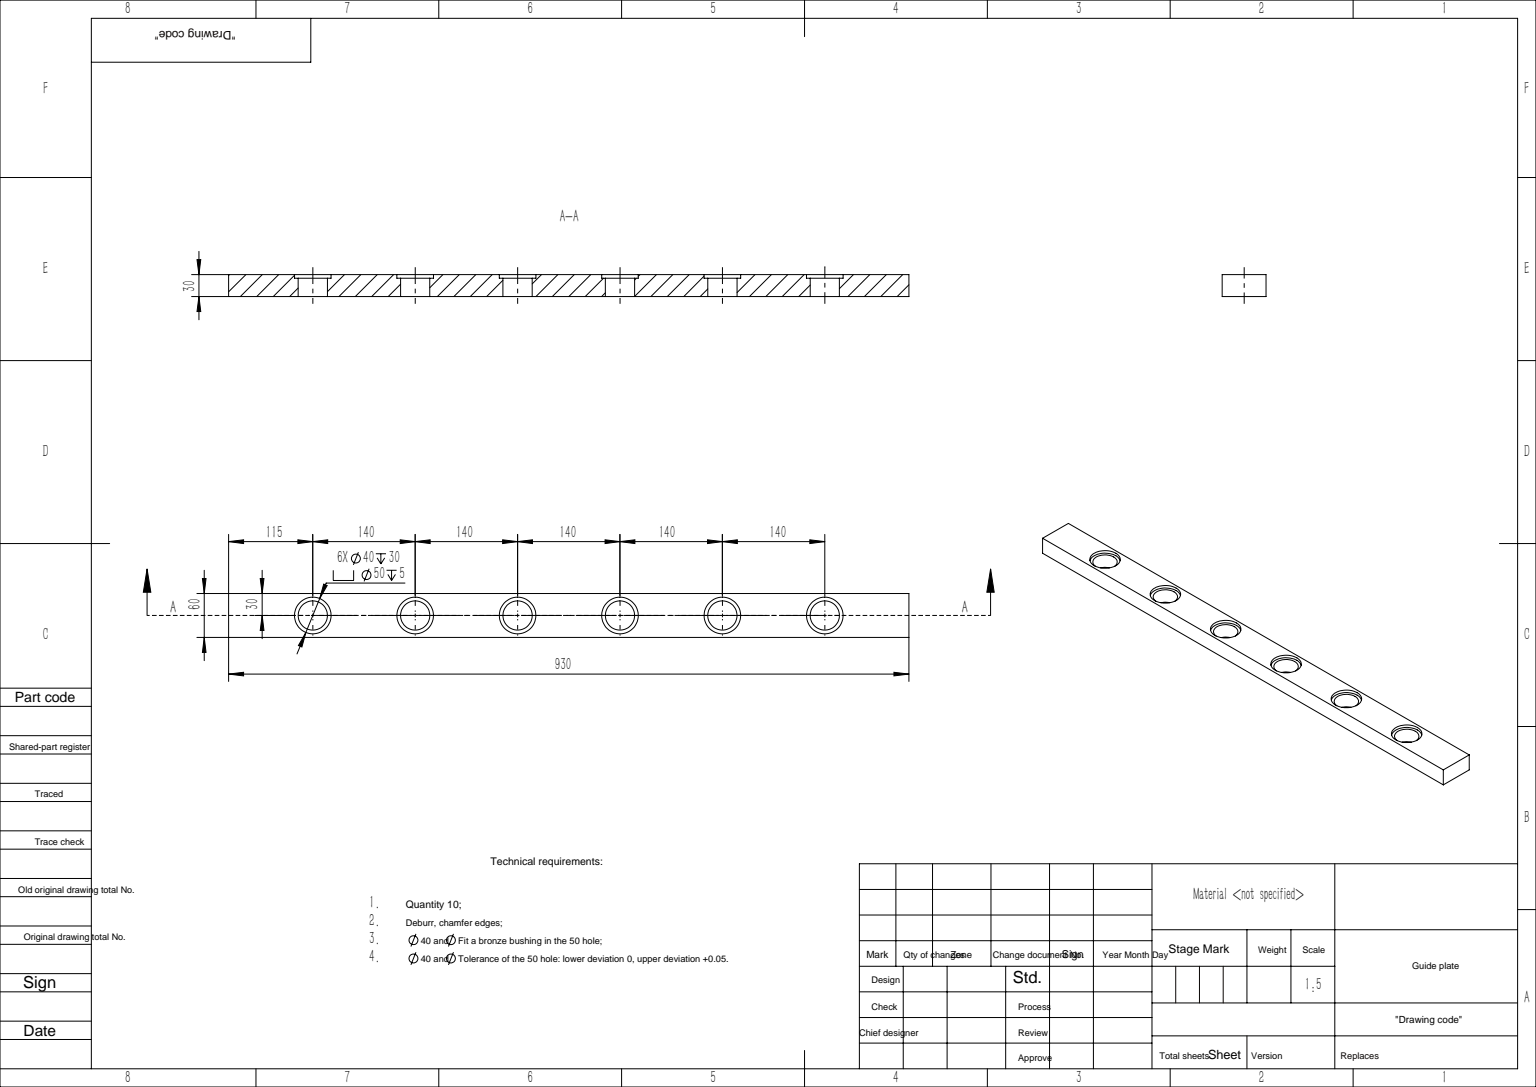
from build123d import *

# Parameters (mm, degrees)
SKETCH_1_W             = 930
SKETCH_1_H             = 60
EXTRUDE_1_DEPTH        = 30
PATTERN_LINEAR_1_COUNT = 6
PATTERN_LINEAR_1_PITCH = 140


with BuildPart() as part:
    # 草图1 → 凸台-拉伸1 (new body)
    with BuildSketch(Plane(origin=(0, 0, 0), x_dir=(1, 0, 0), z_dir=(0, 1, 0))):
        Rectangle(SKETCH_1_W, SKETCH_1_H)
    extrude(amount=EXTRUDE_1_DEPTH)

    # 草图3 → 切除-旋转1 (revolve, cut)
    with BuildSketch(Plane.XY, mode=Mode.PRIVATE) as cut_revolve_1_sk:
        Polygon((350, 30), (375, 30), (375, 25), (370, 25), (370, 0), (350, 0), align=None)
    cut_revolve_1 = revolve(cut_revolve_1_sk.sketch.rotate(Axis((350, 0, 0), (0, 1, 0)), 90), axis=Axis((350, 0, 0), (0, 1, 0)), mode=Mode.SUBTRACT)

    # 阵列(线性)1: 切除-旋转1 ×6
    with Locations(*[(-i * PATTERN_LINEAR_1_PITCH, 0, 0) for i in range(1, PATTERN_LINEAR_1_COUNT)]):
        add(cut_revolve_1, mode=Mode.SUBTRACT)


solid = part.part
